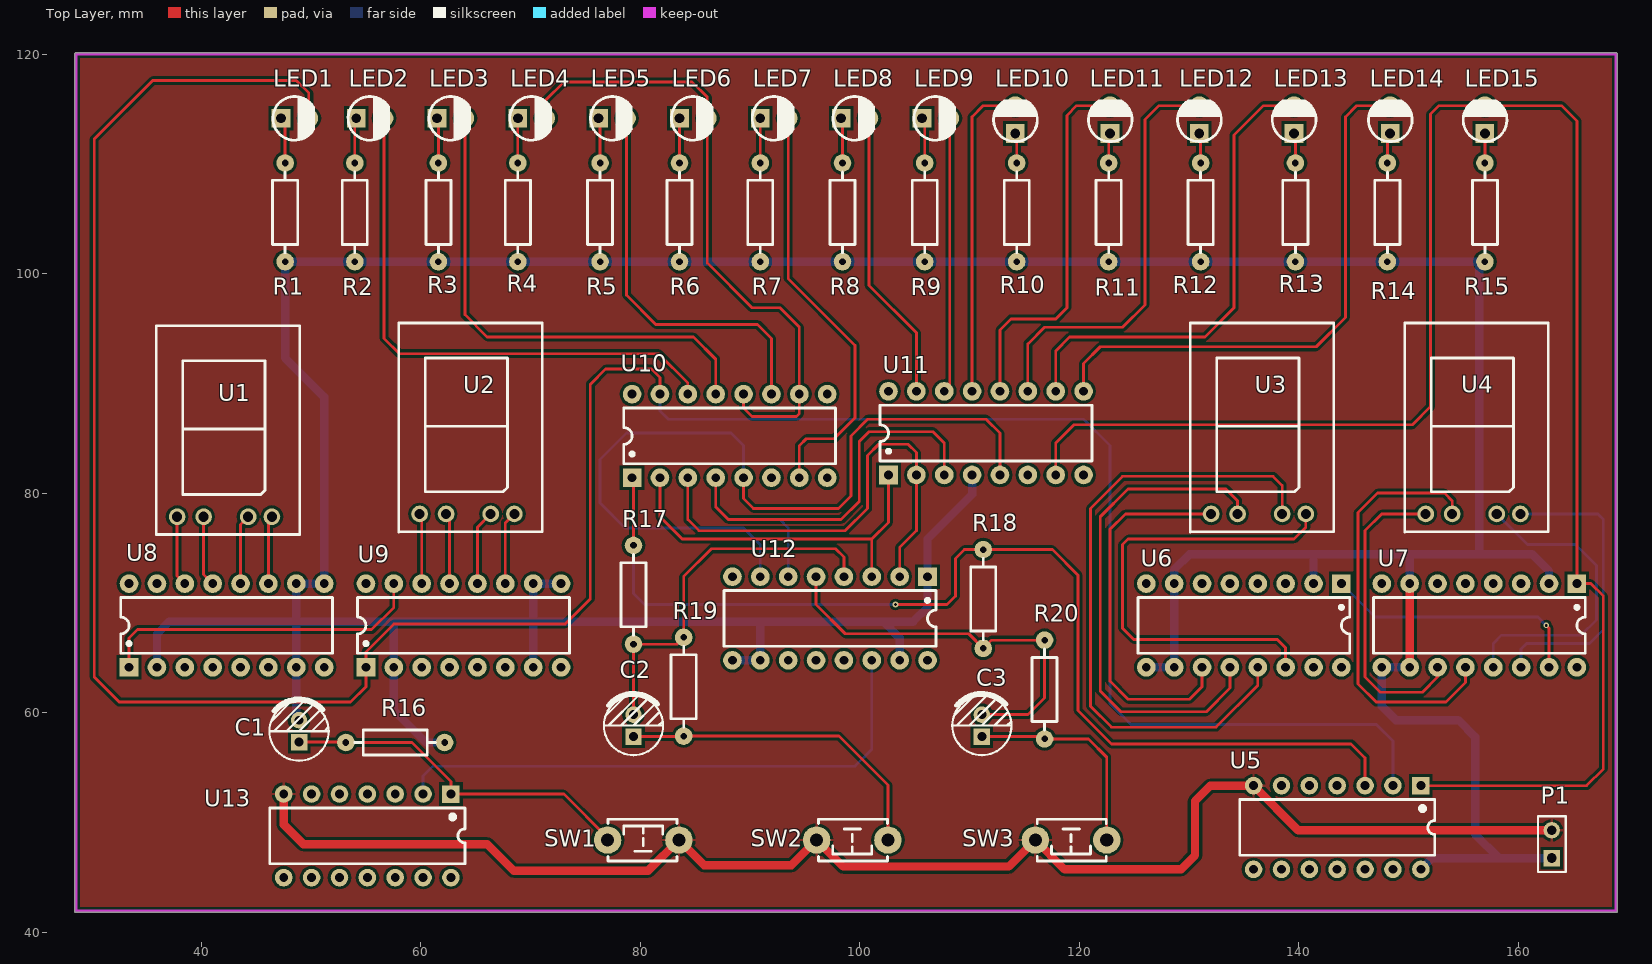
[diagram p0: Top Layer view]
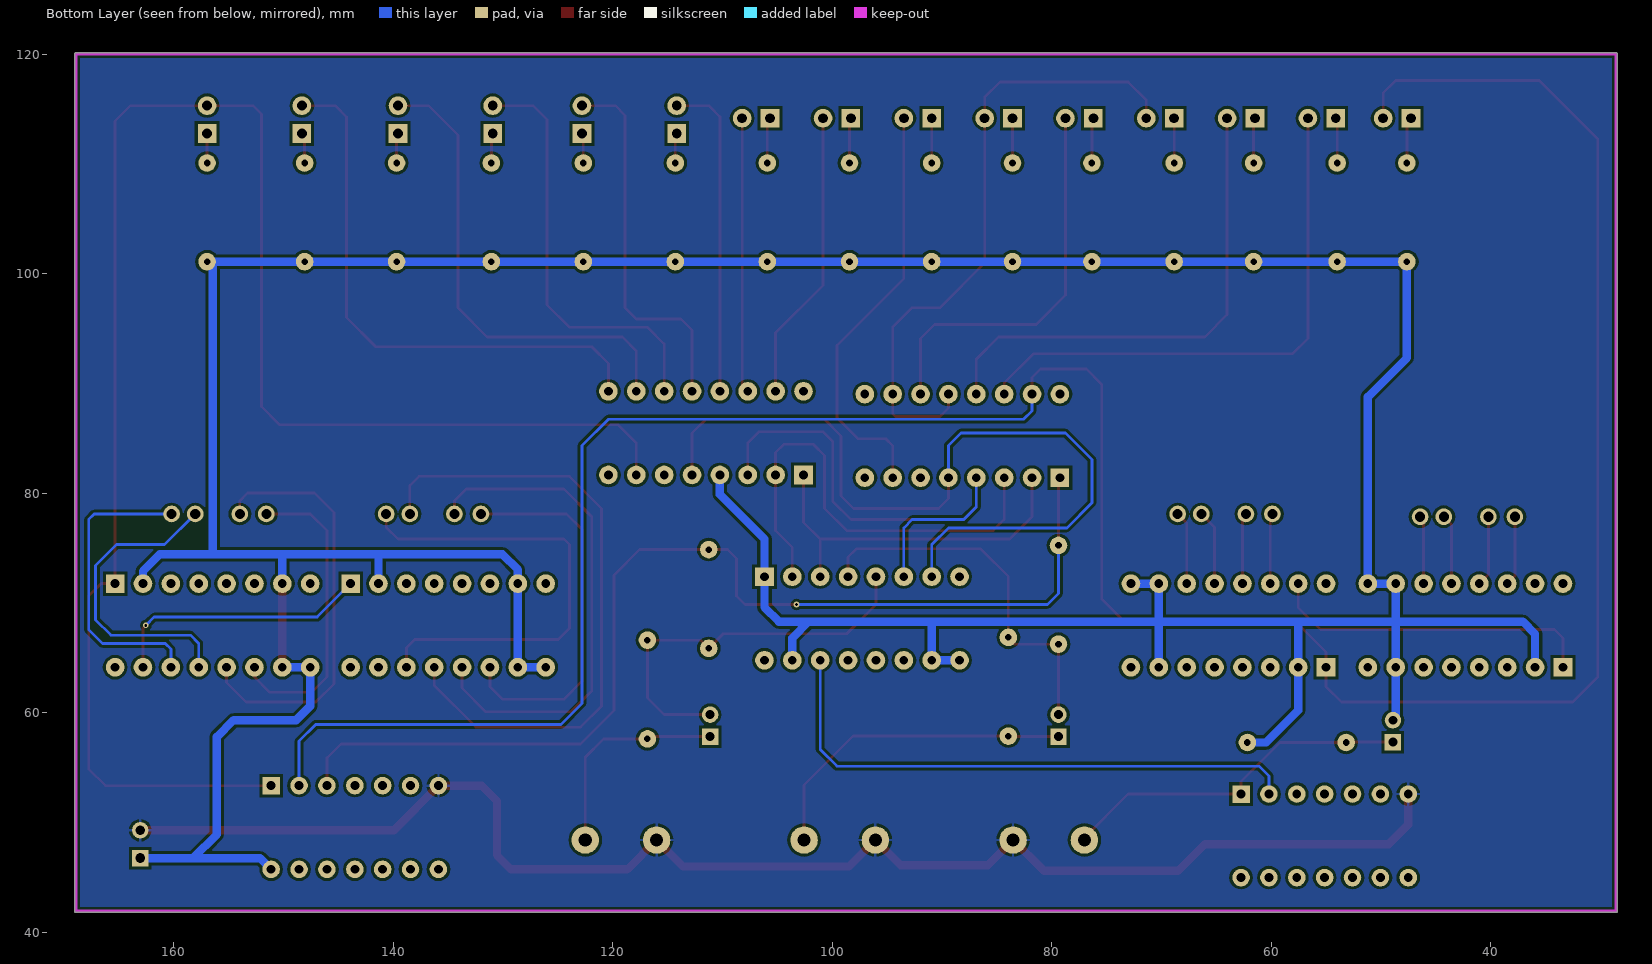
[diagram p1: Bottom Layer view, seen from below]
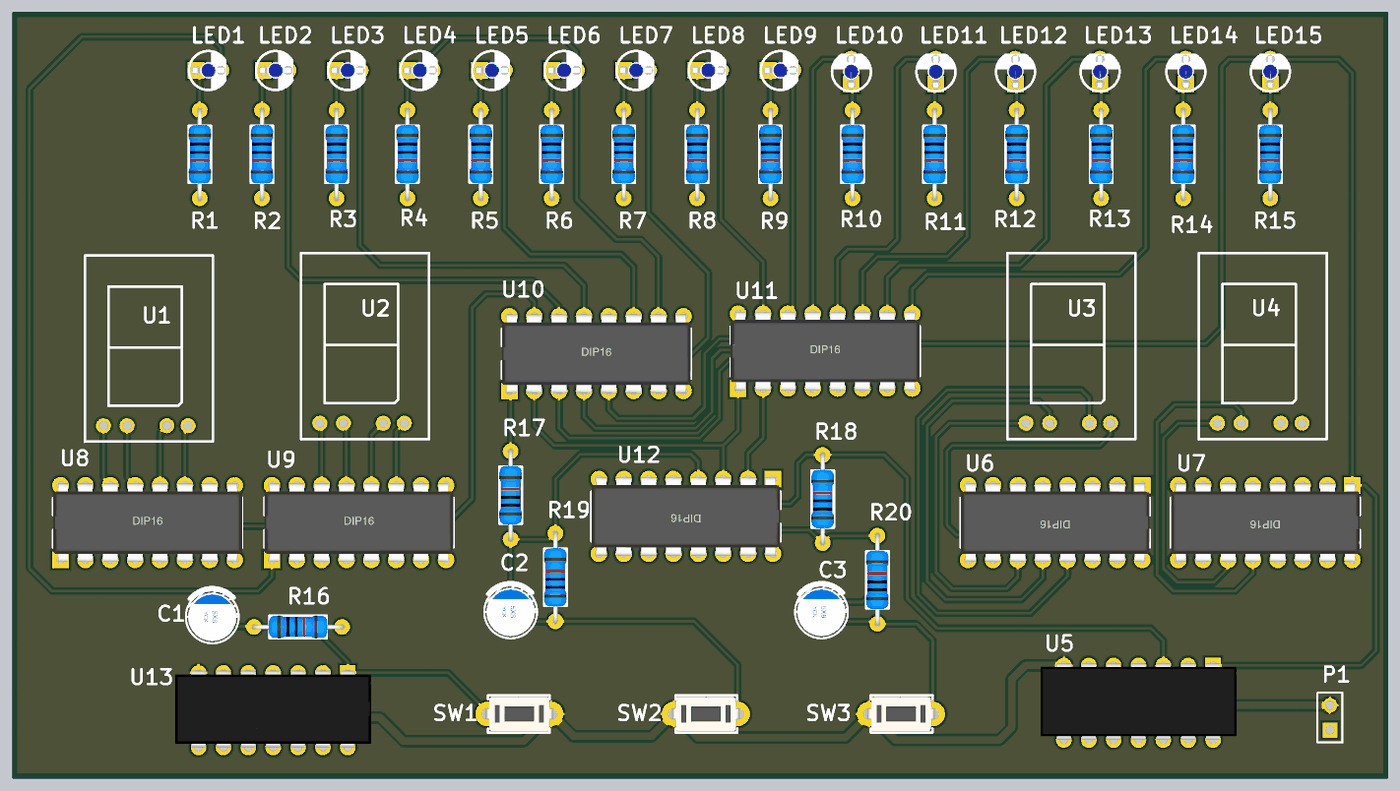
[diagram p2: 3D render of the assembled board from above, using the file's embedded part models]
# Altium PCB MISC80657.PcbDoc
Units mm, origin at the board's own origin, x right, y up, seen from the top; angles counter-clockwise.
Board outline 140.59 x 78.36 mm, 2 copper layers (Top Layer, Bottom Layer); 55 components, 61 nets, 240 pads, 2 vias.

## Layer stack, top to bottom (the 12.6 mil dielectric is the usual default, probably not edited)
Top Solder: solder mask 0.0102, Solder Resist, Dk 3.5
Top Layer: signal copper 0.0356
Dielectric 1: dielectric 0.32, FR-4, Dk 4.8
Bottom Layer: signal copper 0.0356
Bottom Solder: solder mask 0.0102, Solder Resist, Dk 3.5

## Board outline
28.575,41.783 cw(c28.575,41.91) 28.448,41.91 28.448,120.015 cw(c28.575,120.015) 28.575,120.142 168.91,120.142 cw(c168.91,120.015) 169.037,120.015 169.037,41.91 cw(c168.91,41.91) 168.91,41.783

## Design rules (kind name [scope] priority, off if disabled: settings)
Clearance [All] p1: gap=0.254
MinimumSolderMaskSliver [All] p1: minsoldermaskwidth=0
PolygonConnect [All] p1: connectstyle=Relief reliefconductorwidth=0.254 reliefentries=4 polygonreliefangle="90 Angle" airgapwidth=0.254
RoutingVias [All] p1: holewidth=0.711 width=1.27 viastyle="Through Hole" minholewidth=0.711 minwidth=1.27 maxholewidth=0.711 maxwidth=1.27
SilkToSilkClearance [All] p1: silktosilkclearance=0
SilkToSolderMaskClearance [IsPad] p1: minsilkscreentomaskgap=0 clearancetoexposedcopper=TRUE
SolderMaskExpansion [All] p1: expansion=0.102
Width [All] p1: maxlimit=0.762 minlimit=0.254 preferedwidth=0.254
27 further rules are at their usual default settings.

## Components (designator, comment, footprint, x,y, rotation, side; value= is the part's Value field where it differs from the comment)
C1 "Cap" "CS 2.0*5*8 - C" 48.895,58.309 r270 top
C2 "Cap" "CS 2.0*5*8 - C" 79.375,58.817 r270 top
C3 "Cap" "CS 2.0*5*8 - C" 111.125,58.817 r270 top
LED1 "LED1" "LED 3MM-B" 48.514,114.173 r0 top
LED2 "LED2" "LED 3MM-B" 55.372,114.173 r0 top
LED3 "LED3" "LED 3MM-B" 62.738,114.173 r0 top
LED4 "LED4" "LED 3MM-B" 70.104,114.173 r0 top
LED5 "LED1" "LED 3MM-B" 77.47,114.173 r0 top
LED6 "LED1" "LED 3MM-B" 84.836,114.173 r0 top
LED7 "LED1" "LED 3MM-B" 92.202,114.173 r0 top
LED8 "LED1" "LED 3MM-B" 99.568,114.173 r0 top
LED9 "LED1" "LED 3MM-B" 106.934,114.173 r0 top
LED10 "LED1" "LED 3MM-B" 114.173,114.046 r90 top
LED11 "LED1" "LED 3MM-B" 122.809,114.046 r90 top
LED12 "LED1" "LED 3MM-B" 130.937,114.046 r90 top
LED13 "LED1" "LED 3MM-B" 139.573,114.046 r90 top
LED14 "LED1" "LED 3MM-B" 148.336,114.046 r90 top
LED15 "LED1" "LED 3MM-B" 156.972,114.046 r90 top
P1 "Header 2" HDR1X2 163.068,46.736 r90 top
R1 "" "RS 1/4W" 47.625,105.592 r270 top
R2 "Res1" "RS 1/4W" 53.975,105.592 r270 top
R3 "Res1" "RS 1/4W" 61.595,105.592 r270 top
R4 "Res1" "RS 1/4W" 68.834,105.592 r270 top
R5 "Res1" "RS 1/4W" 76.327,105.592 r270 top
R6 "Res1" "RS 1/4W" 83.566,105.592 r270 top
R7 "Res1" "RS 1/4W" 90.932,105.592 r270 top
R8 "Res1" "RS 1/4W" 98.425,105.592 r270 top
R9 "Res1" "RS 1/4W" 105.918,105.592 r270 top
R10 "Res1" "RS 1/4W" 114.3,105.592 r270 top
R11 "Res1" "RS 1/4W" 122.682,105.592 r270 top
R12 "Res1" "RS 1/4W" 131.064,105.592 r270 top
R13 "Res1" "RS 1/4W" 139.7,105.592 r270 top
R14 "Res1" "RS 1/4W" 148.082,105.592 r270 top
R15 "Res1" "RS 1/4W" 156.972,105.592 r270 top
R16 "10k" "RS 1/4W" 57.658,57.277 r0 top
R17 "Res1" "RS 1/4W" 79.375,70.739 r90 top
R18 "Res1" "RS 1/4W" 111.252,70.358 r90 top
R19 "Res1" "RS 1/4W" 83.947,62.357 r90 top
R20 "" "RS 1/4W" 116.84,62.103 r90 top
SW1 "3x6x5" "TSW DIP-3*6*4.3" 80.264,48.387 r0 top
SW2 "3x6x5" "TSW DIP-3*6*4.3" 99.314,48.387 r180 top
SW3 "3x6x5" "TSW DIP-3*6*4.3" 119.253,48.387 r180 top
U1 "LCD1" DCD-HEX 42.418,85.725 r0 top
U2 "LCD1" DCD-HEX 64.516,85.979 r0 top
U3 "LCD1" DCD-HEX 136.652,85.979 r0 top
U4 "LCD1" DCD-HEX 156.21,85.979 r0 top
U5 "SN74LS08D" DIP14 151.13,53.34 r270 top
U6 "SN74LS160AD" DIP16 135.001,67.945 r270 top
U7 "SN74LS160AD" DIP16 156.464,67.945 r270 top
U8 "SN74LS160AD" DIP16 42.291,67.945 r90 top
U9 "SN74LS160AD" DIP16 63.881,67.945 r90 top
U10 "SN74LS138D" DIP16 88.138,85.217 r90 top
U11 "SN74LS138D" DIP16 111.506,85.471 r90 top
U12 "SN74LS193D" DIP16 97.282,68.58 r270 top
U13 "SN74LS04D" DIP14 62.738,52.578 r270 top

## Footprints (in the part's own frame and the unit in brackets; to place one, negate y for a bottom-side part, rotate by r counter-clockwise, add the part's x,y. Pads: shape width x height; smd on the part's side, far side on the other; paste and mask are expansions set on the pad)
"CS 2.0*5*8 - C" [mm] "脚距2mm , 直径5mm , 高8mm"
  rect 1.5x1.5 hole 0.8: 1(1,0)
  round 1.5 hole 0.8: 2(-1,0)
  silkscreen extent -2.96,-2.7 2.7,2.7, body extent -2.5,-2.5 2.5,2.5, height 8.02
DCD-HEX [mil]
  round 60 hole 36 paste+0 mask+2: 1(-182.5,-310) 2(-87.5,-310)
  round 60 hole 36 paste+0 mask+4: 3(72.5,-310) 4(157.5,-310)
  silkscreen extent -258,-375 258,375
DIP14 [mm]
  rect 1.6x1.6 hole 0.813: 1(0,0)
  round 1.6 hole 0.813: 2(0,-2.54) 3(0,-5.08) 4(0,-7.62) 5(0,-10.16) 6(0,-12.7) 7(0,-15.24) 8(7.62,-15.24) 9(7.62,-12.7) 10(7.62,-10.16) 11(7.62,-7.62) 12(7.62,-5.08) 13(7.62,-2.54) 14(7.62,0)
  silkscreen extent 1.27,-16.51 6.35,1.27, body extent -0.25,-17.62 7.62,2.38, height 5.1
DIP16 [mm]
  rect 1.7x1.7 hole 0.8: 1(-3.81,8.89)
  round 1.7 hole 0.8: 2(-3.81,6.35) 3(-3.81,3.81) 4(-3.81,1.27) 5(-3.81,-1.27) 6(-3.81,-3.81) 7(-3.81,-6.35) 8(-3.81,-8.89) 9(3.81,-8.89) 10(3.81,-6.35) 11(3.81,-3.81) 12(3.81,-1.27) 13(3.81,1.27) 14(3.81,3.81) 15(3.81,6.35) 16(3.81,8.89)
  silkscreen extent -2.54,-9.65 2.54,9.65, body extent -4.02,-9.65 4.02,9.65, height 4.45
HDR1X2 [mm] "Connector; Header; 2 Position"
  rect 1.5x1.5 hole 0.9: 1(0,0)
  round 1.5 hole 0.9: 2(2.54,0)
  silkscreen extent -1.27,-1.27 3.81,1.27
"LED 3MM-B" [mm] "蓝色3mm直插LED"
  rect 1.7x1.7 hole 0.9: 1(-1.27,0)
  round 1.7 hole 0.9: 2(1.27,0)
  silkscreen extent -2.01,-2 1.72,1.98, body extent -1.95,-1.95 1.64,1.95, height 5.55
"RS 1/4W" [mm] "直插色环电阻，脚距9mm，直径2.3mm"
  round 1.6 hole 0.6: 1(-4.5,0) 2(4.5,0)
  silkscreen extent -3.68,-1.14 3.68,1.14, body extent -4.72,-1.16 4.73,1.16, height 2.32
"TSW DIP-3*6*4.3" [mm] "3*6*4.3mm"
  round 2.5 hole 1.2: 1(3.25,0) 2(-3.25,0)
  silkscreen extent -3.21,-1.9 3.09,1.9, body extent -3.91,-1.75 3.91,1.75, height 4.31

## Part data
C1 C2 C3: "Capacitor"
LED1 LED2 LED4 LED5 LED6 LED7 LED8 LED9 LED10 LED11 LED12 LED13 LED14 LED15: library part LED3, "Typical BLUE SiC LED"
LED3: "Typical BLUE SiC LED"
P1: "Header, 2-Pin"
R1 R16 R20: library part Res1, "Resistor"
R2 R3 R4 R5 R6 R7 R8 R9 R10 R11 R12 R13 R14 R15 R17 R18 R19: "Resistor"
SW1 SW2 SW3: library part "TSW 3x6", "3x6 tactile switch"
U5: "Quad 2-Input AND Gate"
U6 U7 U8 U9: "BCD Decade Counter"
U10 U11: "1-of-8 Decoder/Demultiplexer"
U12: "Presettable 4-Bit Binary Up/Down Counter"
U13: "Hex Inverter"

## Via types
v1: diameter 0.508, hole 0.254, Top Layer to Bottom Layer, 2 vias

## Nets (pads, with @x,y where several pads share a name; then routed paths per layer and width w, separated by ;. In a path a pad name is that pad's centre, name@x,y a point inside that pad or via, vN(x,y) a via of type N, cw(c..) or ccw(c..) an arc to the next point about the centre after c; other vN are vias at no path point)
GND: P1.2 SW1.1 SW2.1 SW3.1 U5.7 U13.7 | length 134
  Top Layer w0.762: U13.7 47.498,49.784 49.276,48.006 66.04,48.006 68.453,45.593 80.72,45.593 SW1.1 85.8,46.101 93.778,46.101 SW2.1 98.477,45.974 113.59,45.974 SW3.1 118.67,45.72 129.286,45.72 130.556,46.99 130.556,51.943 131.953,53.34 U5.7 139.954,49.276 P1.2
NetC1_1: C1.1 R16.1 SW1.2 U13.1 | length 32.6
  Top Layer w0.254: C1.1 53.126,57.309 R16.1 59.182,57.277 62.738,53.721 U13.1 73.025,52.578 77.014,48.589 SW1.2
NetC2_1: C2.1 R19.1 SW2.2 | length 30.1
  Top Layer w0.254: C2.1 83.907,57.817 R19.1 98.099,57.857 102.564,53.392 SW2.2
NetC2_2: C2.2 R17.1 R19.2 U12.4 | length 34.5
  Top Layer w0.254: C2.2 R17.1 83.329,66.239 R19.2 83.947,72.39 86.487,74.93 97.79,74.93 98.552,74.168 U12.4
NetC3_1: C3.1 R20.1 SW3.2 | length 19.7
  Top Layer w0.254: C3.1 116.626,57.817 R20.1 120.832,57.603 122.503,55.932 SW3.2
NetC3_2: C3.2 R18.1 R20.2 U12.5 | length 36.9
  Top Layer w0.254: U12.5 96.012,69.85 98.679,67.183 109.927,67.183 R18.1 111.997,66.603 R20.2 116.84,61.341 115.316,59.817 C3.2
NetLED1_1: LED1.1 R1.1 | length 4.2
  Top Layer w0.254: LED1.1 47.625,113.792 R1.1
NetLED1_2: LED1.2 U5.2 U9.1 U10.15 | length 252.4
  Top Layer w0.254: LED1.2 49.784,116.459 48.641,117.602 35.56,117.602 30.226,112.268 30.226,63.246 32.512,60.96 53.594,60.96 54.991,62.357 U9.1 54.991,65.532 57.531,68.072 73.152,68.072 75.438,70.358 75.438,89.916 76.835,91.313 81.026,91.313 81.788,90.551 U10.15
  Bottom Layer w0.254: U10.15 81.788,87.503 82.55,86.741 120.396,86.741 122.809,84.328 122.809,60.833 124.714,58.928 147.066,58.928 148.59,57.404 U5.2
NetLED2_1: LED2.1 R2.1 | length 4.1
  Top Layer w0.254: R2.1 53.975,114.046 LED2.1
NetLED2_2: LED2.2 U10.14 | length 50.5
  Top Layer w0.254: LED2.2 56.642,94.107 58.039,92.71 81.661,92.71 84.328,90.043 U10.14
NetLED3_1: LED3.1 R3.1 | length 4.1
  Top Layer w0.254: LED3.1 61.595,114.046 R3.1
NetLED3_2: LED3.2 U10.13 | length 45.6
  Top Layer w0.254: LED3.2 64.008,96.266 66.04,94.234 84.836,94.234 86.868,92.202 U10.13
NetLED4_1: LED4.1 R4.1 | length 4.1
  Top Layer w0.254: R4.1 LED4.1
NetLED4_2: LED4.2 LED6.2 U10.10 U10.12 | length 58.2
  Top Layer w0.254: LED4.2 71.374,115.824 73.025,117.475 84.709,117.475 86.106,116.078 LED6.2 86.106,100.965 90.17,96.901 92.71,96.901 94.488,95.123 U10.10 94.488,87.249 94.234,86.995 90.17,86.995 89.408,87.757 U10.12
NetLED5_1: LED5.1 R5.1 | length 4.1
  Top Layer w0.254: LED5.1 76.327,114.046 R5.1
NetLED5_2: LED5.2 U10.11 | length 36
  Top Layer w0.254: LED5.2 78.74,98.044 81.407,95.377 90.678,95.377 91.948,94.107 U10.11
NetLED6_1: LED6.1 R6.1 | length 4.1
  Top Layer w0.254: R6.1 LED6.1
NetLED7_1: LED7.1 R7.1 | length 4.1
  Top Layer w0.254: R7.1 LED7.1
NetLED7_2: LED7.2 U10.7 | length 38.9
  Top Layer w0.254: LED7.2 93.472,99.568 99.568,93.472 99.568,86.868 97.663,84.963 95.123,84.963 94.488,84.328 U10.7
NetLED8_1: LED8.1 R8.1 | length 4.1
  Top Layer w0.254: LED8.1 98.425,114.046 R8.1
NetLED8_2: LED8.2 U11.15 | length 26.7
  Top Layer w0.254: LED8.2 100.838,98.933 105.156,94.615 U11.15
NetLED9_1: LED9.1 R9.1 | length 4.2
  Top Layer w0.254: LED9.1 105.918,113.919 R9.1
NetLED9_2: LED9.2 U11.14 | length 25.1
  Top Layer w0.254: U11.14 108.204,89.789 LED9.2
NetLED10_1: LED10.1 R10.1 | length 2.7
  Top Layer w0.254: LED10.1 114.3,112.649 R10.1
NetLED10_2: LED10.2 U11.13 | length 29.4
  Top Layer w0.254: U11.13 110.236,114.3 111.252,115.316 LED10.2
NetLED11_1: LED11.1 R11.1 | length 2.7
  Top Layer w0.254: R11.1 122.682,112.649 LED11.1
NetLED11_2: LED11.2 U11.12 | length 34.4
  Top Layer w0.254: U11.12 112.776,94.869 113.792,95.885 117.856,95.885 118.872,96.901 118.872,114.427 119.761,115.316 LED11.2
NetLED12_1: LED12.1 R12.1 | length 2.7
  Top Layer w0.254: LED12.1 131.064,112.649 R12.1
NetLED12_2: LED12.2 U11.11 | length 38.8
  Top Layer w0.254: U11.11 115.316,93.599 116.84,95.123 123.952,95.123 125.984,97.155 125.984,114.046 127.254,115.316 LED12.2
NetLED13_1: LED13.1 R13.1 | length 2.7
  Top Layer w0.254: LED13.1 139.7,112.649 R13.1
NetLED13_2: LED13.2 U11.10 | length 43.9
  Top Layer w0.254: U11.10 117.856,92.964 119.126,94.234 131.445,94.234 134.112,96.901 134.112,112.649 136.779,115.316 LED13.2
NetLED14_1: LED14.1 R14.1 | length 2.8
  Top Layer w0.254: R14.1 148.082,112.522 LED14.1
NetLED14_2: LED14.2 U11.9 | length 50.9
  Top Layer w0.254: U11.9 120.396,91.821 121.92,93.345 141.605,93.345 144.272,96.012 144.272,114.3 145.288,115.316 LED14.2
NetLED15_1: LED15.1 R15.1 | length 2.7
  Top Layer w0.254: R15.1 LED15.1
NetLED15_2: LED15.2 U5.1 U7.1 U11.7 | length 157.4
  Top Layer w0.254: U11.7 117.856,84.582 119.507,86.233 150.368,86.233 152.019,87.884 152.019,114.554 152.781,115.316 LED15.2 163.957,115.316 165.354,113.919 U7.1 166.624,71.755 167.767,70.612 167.767,54.864 166.243,53.34 U5.1
NetR17_2: R17.2 R18.2 U5.3 U10.1 | length 99.4
  Top Layer w0.254: U10.1 79.375,81.28 R17.2 ; v1(103.251,69.85) 107.95,69.85 108.712,70.612 108.712,74.041 109.529,74.858 R18.2 117.547,74.858 119.888,72.517 119.888,60.198 122.936,57.15 144.78,57.15 146.05,55.88 U5.3
  Bottom Layer w0.254: R17.2 79.375,70.866 80.391,69.85 v1(103.251,69.85)
NetU1_1: U1.1 U8.14 | length 6.4
  Top Layer w0.254: U1.1 37.782,72.453 U8.14
NetU1_2: U1.2 U8.13 | length 6.4
  Top Layer w0.254: U1.2 40.195,72.581 U8.13
NetU1_3: U1.3 U8.12 | length 6.4
  Top Layer w0.254: U8.12 43.561,77.153 U1.3
NetU1_4: U1.4 U8.11 | length 6.2
  Top Layer w0.254: U8.11 46.101,77.534 U1.4
NetU2_1: U2.1 U9.14 | length 6.4
  Top Layer w0.254: U2.1 60.071,77.915 U9.14
NetU2_2: U2.2 U9.13 | length 6.5
  Top Layer w0.254: U2.2 62.611,77.787 U9.13
NetU2_3: U2.3 U9.12 | length 6.8
  Top Layer w0.254: U9.12 65.151,76.898 U2.3
NetU2_4: U2.4 U9.11 | length 6.7
  Top Layer w0.254: U9.11 67.691,77.279 U2.4
NetU3_1: U3.1 U6.11 | length 34.9
  Top Layer w0.254: U6.11 131.191,62.357 130.048,61.214 124.46,61.214 122.809,62.865 122.809,76.708 124.206,78.105 U3.1
NetU3_2: U3.2 U6.12 | length 46.5
  Top Layer w0.254: U6.12 133.731,62.23 131.572,60.071 123.825,60.071 121.92,61.976 121.92,77.851 124.46,80.391 133.35,80.391 134.429,79.311 U3.2
NetU3_3: U3.3 U6.13 | length 58.9
  Top Layer w0.254: U6.13 136.271,62.484 132.461,58.674 122.936,58.674 121.031,60.579 121.031,78.613 123.952,81.534 137.668,81.534 138.493,80.709 U3.3
NetU3_4: U3.4 U6.14 | length 43.6
  Top Layer w0.254: U6.14 138.811,65.913 138.049,66.675 124.968,66.675 123.952,67.691 123.952,75.311 124.46,75.819 139.573,75.819 140.653,76.898 U3.4
NetU4_1: U4.1 U7.11 | length 28.1
  Top Layer w0.254: U4.1 147.574,78.105 146.05,76.581 146.05,63.246 147.447,61.849 151.257,61.849 152.654,63.246 U7.11
NetU4_2: U4.2 U7.12 | length 39
  Top Layer w0.254: U4.2 153.987,79.311 153.289,80.01 147.193,80.01 145.415,78.232 145.415,62.611 147.066,60.96 153.416,60.96 155.194,62.738 U7.12
NetU4_3: U4.3 U7.13 | length 28.4
  Bottom Layer w0.254: U7.13 157.734,66.294 158.496,67.056 165.735,67.056 167.132,68.453 167.132,73.406 165.227,75.311 160.845,75.311 U4.3
NetU4_4: U4.4 U7.14 | length 27.7
  Bottom Layer w0.254: U4.4 167.259,78.105 167.767,77.597 167.767,67.564 166.497,66.294 160.782,66.294 160.274,65.786 U7.14
NetU6_1: U6.1 U7.15 | length 24.2
  Top Layer w0.254: v1(162.56,67.945) 162.814,67.691 U7.15
  Bottom Layer w0.254: U6.1 146.939,68.707 161.798,68.707 v1(162.56,67.945)
NetU8_1: U8.1 U9.15 | length 30.1
  Top Layer w0.254: U8.1 33.401,66.802 34.163,67.564 55.499,67.564 57.531,69.596 U9.15
NetU10_2: U10.2 U11.1 U12.3 | length 33.6
  Top Layer w0.254: U10.2 81.788,77.851 83.82,75.819 101.092,75.819 ; U12.3 101.092,75.819 ; U11.1 102.616,77.343 101.092,75.819
NetU10_3: U10.3 U11.2 U12.2 | length 43.4
  Top Layer w0.254: U10.3 84.328,77.597 85.344,76.581 98.679,76.581 100.711,78.613 100.711,83.439 101.727,84.455 104.394,84.455 105.156,83.693 U11.2 105.156,76.581 103.632,75.057 U12.2
NetU10_4: U10.4 U11.3 U12.6 | length 48.3
  Top Layer w0.254: U10.4 86.868,78.74 88.011,77.597 98.298,77.597 99.949,79.248 99.949,84.709 100.838,85.598 106.68,85.598 107.696,84.582 U11.3
  Bottom Layer w0.254: U10.4 86.868,78.74 88.011,77.597 92.71,77.597 93.472,76.835 U12.6
NetU10_5: U10.5 U11.5 U12.7 | length 77.1
  Top Layer w0.254: U10.5 89.408,79.502 90.297,78.613 98.044,78.613 99.187,79.756 99.187,85.217 100.711,86.741 111.506,86.741 112.776,85.471 U11.5
  Bottom Layer w0.254: U10.5 89.408,84.328 88.265,85.471 78.74,85.471 76.327,83.058 76.327,79.121 78.613,76.835 89.408,76.835 90.932,75.311 U12.7
NetU12_14: U12.14 U13.2 | length 51.7
  Bottom Layer w0.254: U13.2 60.198,54.229 61.087,55.118 99.568,55.118 101.092,56.642 U12.14
VCC: C1.2 P1.1 R1.2 R2.2 R3.2 R4.2 R5.2 R6.2 R7.2 R8.2 R9.2 R10.2 R11.2 R12.2 R13.2 R14.2 R15.2 R16.2 U5.14 U6.2 U6.7 U6.9 U6.10 U7.2 U7.7 U7.9 U7.10 U8.2 U8.7 U8.9 U8.10 U9.2 U9.7 U9.9 U9.10 U11.4 U12.1 U12.9 U12.10 U12.15 | length 405.7
  Top Layer w0.762: U7.10 U7.7
  Bottom Layer w0.762: U8.2 35.941,67.183 37.05,68.292 48.641,68.292 ; C1.2 48.641,59.563 U8.7 48.641,68.292 ; R16.2 60.452,57.277 57.531,60.198 U9.2 57.531,68.165 57.658,68.292 ; U9.7 70.231,68.038 ; U9.9 U9.10 70.231,68.292 ; U12.9 U12.10 90.932,68.292 ; U12.15 103.632,66.802 102.142,68.292 ; U11.4 110.236,79.883 106.172,75.819 U12.1 106.172,69.596 104.868,68.292 102.142,68.292 ; U6.9 U6.10 U6.7 128.651,73.025 130.048,74.422 141.478,74.422 ; U6.2 141.351,74.295 141.478,74.422 ; U7.10 U7.9 147.574,60.579 148.844,59.309 154.559,59.309 156.083,57.785 156.083,48.895 158.242,46.736 ; U7.7 150.114,74.295 150.241,74.422 ; U5.14 152.146,46.736 158.242,46.736 ; U7.2 162.814,72.898 161.29,74.422 156.464,74.422 ; P1.1 158.242,46.736 ; 48.641,68.292 57.658,68.292 ; 48.641,68.292 U8.10 U8.9 51.181,88.773 47.625,92.329 R1.2 R2.2 R3.2 R4.2 R5.2 R6.2 R7.2 R8.2 R9.2 R10.2 R11.2 R12.2 R13.2 R14.2 R15.2 156.464,100.584 156.464,74.422 ; 57.658,68.292 70.231,68.292 ; 70.231,68.038 70.231,68.292 ; 70.231,68.038 70.485,68.292 90.932,68.292 ; 90.932,68.292 102.142,68.292 ; 141.478,74.422 150.241,74.422 ; 150.241,74.422 156.464,74.422
VDD: U13.14
pads on no net: U5.4 U5.5 U5.6 U5.8 U5.9 U5.10 U5.11 U5.12 U5.13 U6.3 U6.4 U6.5 U6.6 U6.8 U6.15 U6.16 U7.3 U7.4 U7.5 U7.6 U7.8 U7.16 U8.3 U8.4 U8.5 U8.6 U8.8 U8.15 U8.16 U9.3 U9.4 U9.5 U9.6 U9.8 U9.16 U10.6 U10.8 U10.9 U10.16 U11.6 U11.8 U11.16 U12.8 U12.11 U12.12 U12.13 U12.16 U13.3 U13.4 U13.5 U13.6 U13.8 U13.9 U13.10 U13.11 U13.12 U13.13

## Polygon pours and split planes (outlines as drawn)
GND on Bottom Layer "D" (solid, remove dead copper, pour order 4): 25.4,123.444 26.924,124.968 172.212,124.968 172.212,38.354 171.577,37.719 171.196,37.338 27.813,37.338
GND on Top Layer "D" (solid, remove dead copper, pour order 6): 17.653,125.095 170.942,125.095 176.022,120.015 171.831,115.824 171.831,35.56 25.273,35.56 24.384,36.449

## Keep-outs
Keep-Out Layer:
  lines w0.254: 45.085,120.015 168.91,120.015 168.91,41.91 28.575,41.91 28.575,120.015 46.228,120.015